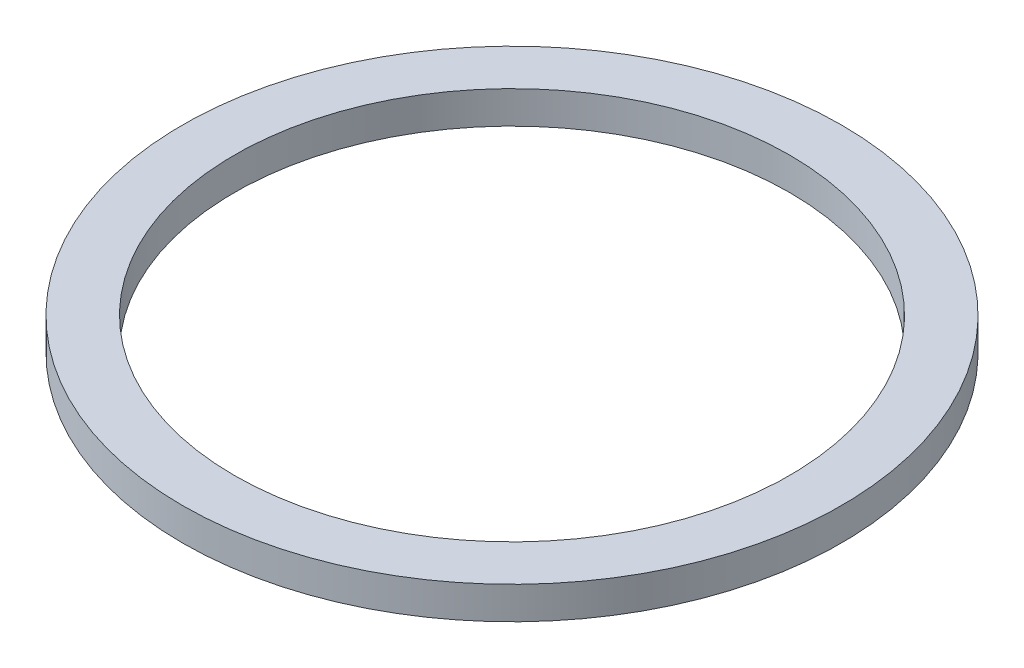
from build123d import *

# Parameters (mm, degrees)
SKETCH1_R           = 27.9
SKETCH1_R_2         = 23.5
BOSS_EXTRUDE1_DEPTH = 2.75


with BuildPart() as part:
    # Sketch1 → Boss-Extrude1 (new body)
    with BuildSketch(Plane(origin=(0, 0, 0), x_dir=(1, 0, 0), z_dir=(0, 1, 0))):
        with Locations(Location((0, 0, 0), (0, 0, 270))):
            Circle(SKETCH1_R)
        with Locations(Location((0, 0, 0), (0, 0, 270))):
            Circle(SKETCH1_R_2, mode=Mode.SUBTRACT)
    extrude(amount=BOSS_EXTRUDE1_DEPTH)


solid = part.part
